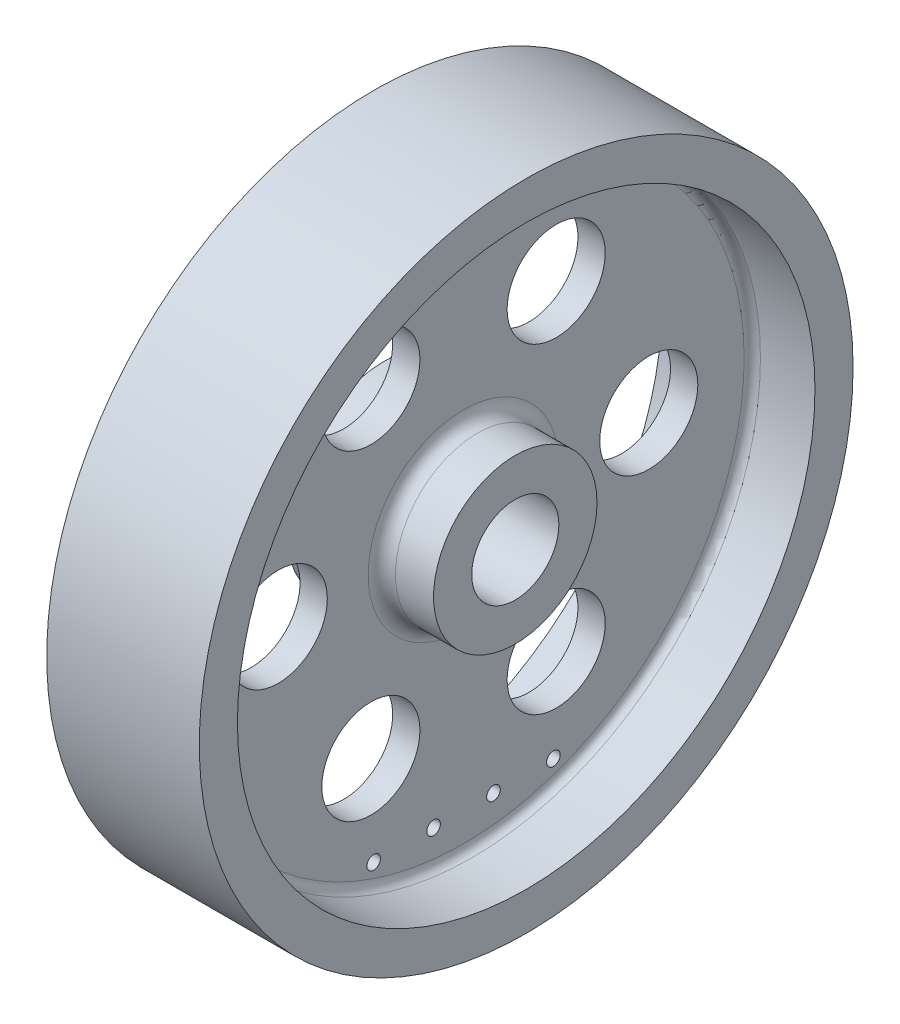
from build123d import *

# Parameters (mm, degrees)
SKETCH4_R          = 90
CUT_EXTRUDE1_DEPTH = 343
CIRPATTERN1_COUNT  = 6
CIRPATTERN2_COUNT  = 3
SKETCH8_R          = 12.5
CUT_EXTRUDE3_DEPTH = 238


with BuildPart() as part:
    # Sketch2 → Revolve1 (revolve)
    with BuildSketch(Plane.XY, mode=Mode.PRIVATE) as revolve1_sk:
        with BuildLine():
            Line((-20, 600), (-20, 530))
            Line((-20, 530), (80, 530))
            ThreePointArc((80, 530), (90.606601718, 525.606601718), (95, 515))
            Line((95, 515), (95, 205))
            ThreePointArc((95, 205), (87.67766953, 187.32233047), (70, 180))
            Line((70, 180), (0, 180))
            Line((0, 180), (0, 105))
            Line((0, 105), (70, 105))
            Line((70, 105), (70, 80))
            Line((70, 80), (240, 80))
            Line((240, 80), (240, 150))
            Line((240, 150), (170, 150))
            ThreePointArc((170, 150), (152.32233047, 157.32233047), (145, 175))
            Line((145, 175), (145, 515))
            ThreePointArc((145, 515), (149.393398282, 525.606601718), (160, 530))
            Line((160, 530), (260, 530))
            Line((260, 530), (260, 600))
            Line((260, 600), (-20, 600))
        make_face()
    revolve(revolve1_sk.sketch.rotate(Axis((225.657059372, 0, 0), (-1, 0, 0)), 90), axis=Axis((225.657059372, 0, 0), (-1, 0, 0)))

    # Sketch4 → Cut-Extrude1 (cut)
    with BuildSketch(Plane(origin=(0, 0, 0), x_dir=(0, 0, -1), z_dir=(1, 0, 0))):
        with Locations(Location((-170, 294.448637287, 0), (0, 0, 180))):
            Circle(SKETCH4_R)
    cut_extrude1 = extrude(amount=CUT_EXTRUDE1_DEPTH, mode=Mode.SUBTRACT)

    # CirPattern1: Cut-Extrude1 ×6 about axis
    cirpattern1_axis = Axis((0, 0, 0), (1, 0, 0))
    for i in range(1, CIRPATTERN1_COUNT):
        add(cut_extrude1.rotate(cirpattern1_axis, i * 360 / CIRPATTERN1_COUNT), mode=Mode.SUBTRACT)

    # Sketch6 → M24 Tapped Hole1 (revolve, cut)
    with BuildSketch(Plane(origin=(0, 114.748366001, 66.25), x_dir=(0, 0, 1), z_dir=(0, 1, 0))):
        Polygon((0, 0), (0, 46.3090365), (10.5, 40), (10.5, 0), align=None)
    m24_tapped_hole1 = revolve(axis=Axis((-6.35, 114.748366001, 66.25), (1, 0, 0)), mode=Mode.SUBTRACT)

    # CirPattern2: M24 Tapped Hole1 ×3 about axis
    cirpattern2_axis = Axis((0, 0, 0), (1, 0, 0))
    for i in range(1, CIRPATTERN2_COUNT):
        add(m24_tapped_hole1.rotate(cirpattern2_axis, i * 360 / CIRPATTERN2_COUNT), mode=Mode.SUBTRACT)

    # Sketch8 → Cut-Extrude3 (cut)
    with BuildSketch(Plane(origin=(0, 0, 0), x_dir=(0, 0, -1), z_dir=(1, 0, 0))):
        with Locations(Location((-55, -462, 0), (0, 0, 180))):
            Circle(SKETCH8_R)
        with Locations(Location((-165, -462, 0), (0, 0, 180))):
            Circle(SKETCH8_R)
        with Locations(Location((55, -462, 0), (0, 0, 180))):
            Circle(SKETCH8_R)
        with Locations(Location((165, -462, 0), (0, 0, 180))):
            Circle(SKETCH8_R)
    extrude(amount=CUT_EXTRUDE3_DEPTH, mode=Mode.SUBTRACT)


solid = part.part
